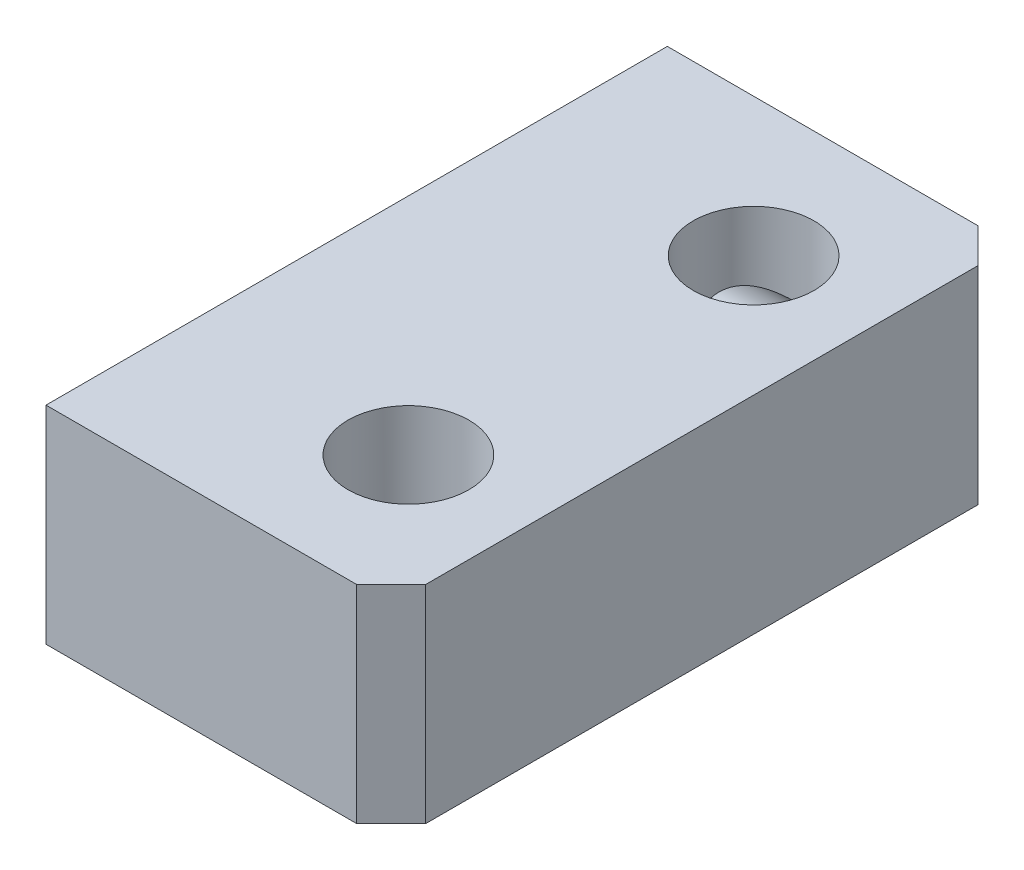
SolidWorks part; units mm, degrees
ref_plane "Front Plane" through (0, 0, 0) normal (0, 0, 1) x (1, 0, 0)
ref_plane "Top Plane" through (0, 0, 0) normal (0, 1, 0) x (1, 0, 0)
ref_plane "Right Plane" through (0, 0, 0) normal (1, 0, 0) x (0, 0, -1)
sketch "Sketch1" plane through (0, 0, 0) normal (0, 1, 0) x (1, 0, 0)
  line L1 (-5, 9) -> (5, 9)
  line L2 (-5, 9) -> (-5, -9)
  line L3 (-5, -9) -> (5, -9)
  line L4 (5, 9) -> (5, -9)
  line L5 (-5, 9) -> (5, -9) construction
  line L6 (-5, -9) -> (5, 9) construction
  point P0 (0, 0)
  dimension "D1" = 10
  dimension "D2" = 18
extrude "Boss-Extrude1" add sketch "Sketch1" along normal blind 6
sketch "Sketch2" plane through (0, 6, 0) normal (0, 1, 0) x (1, 0, 0)
  line L0 (5, -9) -> (5, 9) construction
  line L2 (-5, 0) -> (49995, 0) construction
  line L3 (-5, 9) -> (-5, -9) construction
  circle A0 centre (1.5, 5) radius 1.75
  circle A1 centre (1.5, -5) radius 1.75
  point P9 (-5, 0)
  dimension "D1" = 10
  dimension "D2" = 3.5
  dimension "D3" = 3.5
extrude "Cut-Extrude1" cut sketch "Sketch2" against normal blind 10
chamfer "Chamfer1" distance 1 angle 45 2 edges at (5, 3, 9) (5, 3, -9)
hole_wizard "M2.5 Tapped Hole1" positions "3DSketch1" profile "Sketch3" tap size "M2.5" standard "Gb"
sketch3d "3DSketch1"
  point P0 (-5, 3, -6)
  point P2 (-5, 3, 6)
  dimension "D1" = 12
  dimension "D2" = 3
  dimension "D3" = 3
sketch "Sketch3" plane through (-5, 3, -6) normal (0, 1, 0) x (0, 0, 1)
  line L0 (0, 0) -> (0, 6.9659)
  line L1 (0, 6.9659) -> (1.025, 6.35)
  line L2 (1.025, 6.35) -> (1.025, 0)
  line L5 (1.025, 0) -> (0, 0)
  line L10 (0, 6.9659) -> (-1.025, 6.35) construction
  line L11 (0, -6.35) -> (0, 107.95) construction
  dimension "螺纹孔钻头直径" = 2.05
  dimension "螺纹孔钻头深度" = 6.35
  dimension "导头角度" = 118
cosmetic thread "Cosmetic Thread1" parameters "D1"=5, "D2"=2.5
cosmetic thread "Cosmetic Thread2" parameters "D1"=5, "D2"=2.5
